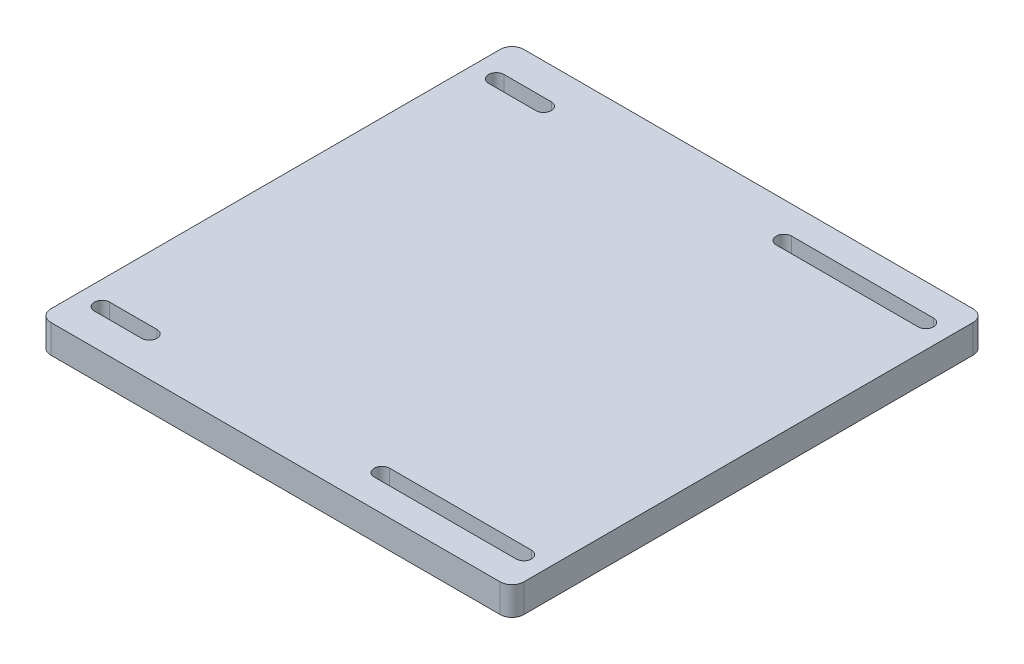
from build123d import *

# Parameters (mm, degrees)
SKETCH_1_W          = 200
SKETCH_1_H          = 200
EXTRUDE_1_DEPTH     = 12
FILLET_1_R          = 5
CUT_EXTRUDE_1_DEPTH = 10


with BuildPart() as part:
    # 草图1 → 凸台-拉伸1 (new body)
    with BuildSketch(Plane(origin=(0, 0, 0), x_dir=(1, 0, 0), z_dir=(0, 1, 0))):
        Rectangle(SKETCH_1_W, SKETCH_1_H)
    extrude(amount=EXTRUDE_1_DEPTH)

    # 圆角1
    fillet_1_edges = [part.edges().sort_by_distance(p)[0] for p in [
        (100, 6, 100),
        (-100, 6, 100),
        (-100, 6, -100),
        (100, 6, -100),
    ]]
    fillet(fillet_1_edges, radius=FILLET_1_R)

    # 草图2 → 切除-拉伸1 (cut)
    with BuildSketch(Plane(origin=(0, 12, 0), x_dir=(1, 0, 0), z_dir=(0, 1, 0))):
        with BuildLine():
            Line((-90, 86.625), (-70, 86.625))
            ThreePointArc((-70, 86.625), (-66.75, 83.375), (-70, 80.125))
            Line((-70, 80.125), (-90, 80.125))
            ThreePointArc((-90, 80.125), (-93.25, 83.375), (-90, 86.625))
        make_face()
        with BuildLine():
            Line((-90, -86.625), (-70, -86.625))
            ThreePointArc((-70, -86.625), (-66.75, -83.375), (-70, -80.125))
            Line((-70, -80.125), (-90, -80.125))
            ThreePointArc((-90, -80.125), (-93.25, -83.375), (-90, -86.625))
        make_face()
        with BuildLine():
            Line((30, 88.25), (90, 88.25))
            ThreePointArc((90, 88.25), (93.25, 85), (90, 81.75))
            Line((90, 81.75), (30, 81.75))
            ThreePointArc((30, 81.75), (26.75, 85), (30, 88.25))
        make_face()
        with BuildLine():
            Line((30, -88.25), (90, -88.25))
            ThreePointArc((90, -88.25), (93.25, -85), (90, -81.75))
            Line((90, -81.75), (30, -81.75))
            ThreePointArc((30, -81.75), (26.75, -85), (30, -88.25))
        make_face()
    extrude(amount=-CUT_EXTRUDE_1_DEPTH, mode=Mode.SUBTRACT)


solid = part.part
